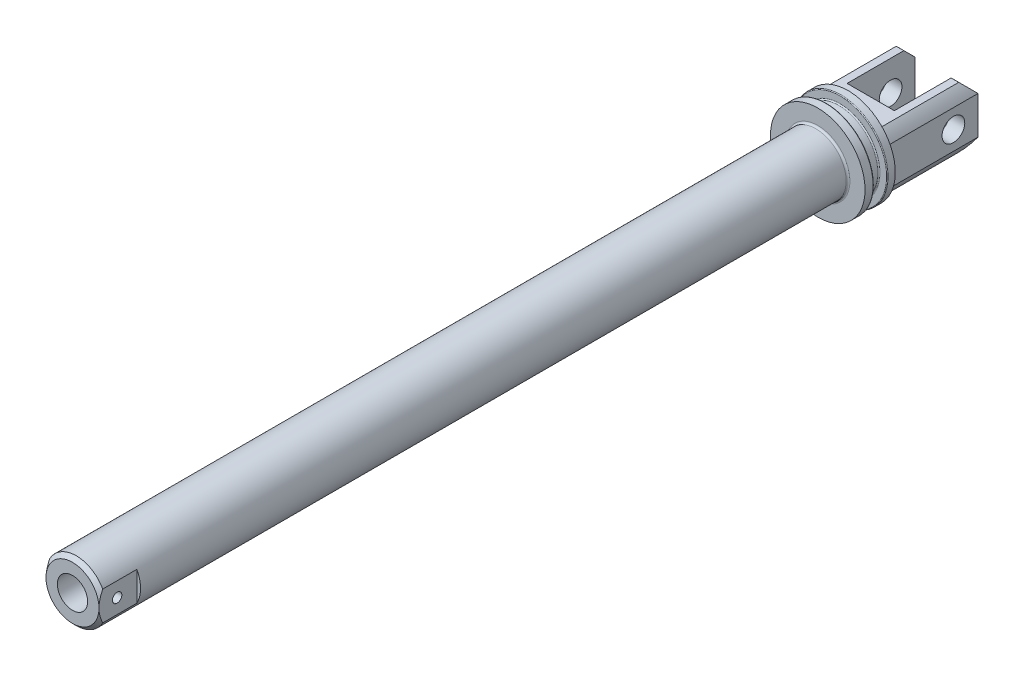
SolidWorks part; units mm, degrees
ref_plane "Front Plane" through (0, 0, 0) normal (0, 0, 1) x (1, 0, 0)
ref_plane "Top Plane" through (0, 0, 0) normal (0, 1, 0) x (1, 0, 0)
ref_plane "Right Plane" through (0, 0, 0) normal (1, 0, 0) x (0, 0, -1)
sketch "Sketch1" plane through (0, 0, 0) normal (0, 0, 1) x (1, 0, 0)
  circle A0 centre (0, 0) radius 8
extrude "Boss-Extrude1" add sketch "Sketch1" along normal blind 197
sketch "Sketch2" plane through (0, 0, 0) normal (0, 0, -1) x (-1, 0, 0)
  circle A0 centre (0, 0) radius 12.5
extrude "Boss-Extrude2" add sketch "Sketch2" along normal blind 8
sketch "Sketch3" plane through (0, 0, 0) normal (0, 1, 0) x (1, 0, 0)
  line L0 (-12.5, 8) -> (-12.5, 0) construction
  line L1 (-12.5, 5.9) -> (-10.25, 5.9)
  line L2 (-12.5, 5.9) -> (-12.5, 2.3)
  line L3 (-12.5, 2.3) -> (-10.25, 2.3)
  line L4 (-10.25, 5.9) -> (-10.25, 2.3)
  line L5 (12.5, 8) -> (-12.5, 8) construction
  line L6 (0, 10.0082) -> (0, -3.7228) construction
  dimension "D1" = 3.6
  dimension "D2" = 2.1
  dimension "D3" = 2.25
revolve "Cut-Revolve1" cut sketch "Sketch3" angle 360 about L6
sketch "Sketch8" plane through (0, 0, -8) normal (0, 0, -1) x (-1, 0, 0)
  circle A0 centre (0, 0) radius 11.5
extrude "Boss-Extrude4" add sketch "Sketch8" along normal blind 24
sketch "Sketch10" plane through (0, 0, 0) normal (0, 1, 0) x (1, 0, 0)
  line L0 (0, 37.7371) -> (0, 5.0633) construction
  line L1 (11.5, 32) -> (-11.5, 32) construction
  line L2 (-6.25, 35.6058) -> (6.25, 35.6058)
  line L3 (-6.25, 35.6058) -> (-6.25, 14)
  line L4 (-6.25, 14) -> (6.25, 14)
  line L5 (6.25, 35.6058) -> (6.25, 14)
  line L6 (-6.25, 35.6058) -> (6.25, 14) construction
  line L7 (-6.25, 14) -> (6.25, 35.6058) construction
  point P3 (0, 24.8029)
  dimension "D1" = 18
  dimension "D2" = 12.5
extrude "Cut-Extrude1" cut sketch "Sketch10" against normal through all both and the other way through all
sketch "Sketch13" plane through (0, 0, -32) normal (0, 0, -1) x (-1, 0, 0)
  line L0 (10.3562, -5) -> (10.3562, 5)
  line L9 (11, 5) -> (10.3562, 4.7073) construction
  line L10 (10.4692, -4.7587) -> (10.3562, -4.7073) construction
  line L11 (-10.3562, -5) -> (-10.3562, 5)
  arc A0 (-10.3562, 5) -> (-10.3562, -5) centre (0, 0) ccw
  arc A1 (10.3562, -5) -> (10.3562, 5) centre (0, 0) ccw
  point P0 (0, 0)
  point P1 (0, 0)
sketch "Sketch11" plane through (0, -11.5, -32) normal (-1, 0, 0) x (0, 0, -1)
  line L1 (-32, -11.5) -> (13.2543, -11.5) construction
  line L7 (1.4984, -3.5) -> (-24, -19.5) construction
  line L8 (1.4984, -19.5) -> (-24, -3.5) construction
  line L9 (0.011, -16.5) -> (-3, -19.5)
  line L11 (-24, -19.5) -> (-24, -26.3966)
  line L12 (-24, -26.3966) -> (1.4984, -26.3966)
  line L13 (1.4984, -19.5) -> (1.4984, -26.3966)
  line L15 (-24, -3.5) -> (-24, 3.3597)
  line L16 (-24, 3.3597) -> (2.7695, 3.3597)
  line L17 (2.7695, -3.5) -> (2.7695, 3.3597)
  line L18 (0, -21.1534) -> (0, -1.8466) construction
  line L19 (1.4984, -19.5) -> (0.011, -19.5)
  line L20 (0.011, -19.5) -> (0.011, -16.5)
  line L21 (-3, -19.5) -> (-24, -19.5)
  line L22 (-3, -3.5) -> (-24, -3.5)
  line L23 (0.011, -6.5) -> (-3, -3.5)
  line L24 (0.011, -3.5) -> (0.011, -6.5)
  line L25 (1.4984, -3.5) -> (0.011, -3.5)
  line L26 (1.4984, -3.5) -> (2.7695, -3.5)
  point P0 (-11.2508, -11.5)
  dimension "D1" = 3
  dimension "D2" = 16
  dimension "D3" = 3
extrude "Cut-Extrude3" cut sketch "Sketch11" against normal through all both and the other way through all
extrude "Cut-Extrude5" cut sketch "Sketch13" against normal blind 24
fillet "Fillet1" radius 0.5 1 edges at (8, 0, 0)
fillet "Fillet2" radius 0.2 2 edges at (-12.5, 0, -5.9) (-12.5, 0, -2.3)
fillet "Fillet3" radius 0.3 2 edges at (-10.25, 0, -2.3) (-10.25, 0, -5.9)
chamfer "Chamfer3" distance 1 angle 45 1 edges at (8, 0, 197)
sketch "Sketch15" plane through (0, 8, 0) normal (0, 1, 0) x (1, 0, 0)
  line L0 (8, -196) -> (8, -0.5) construction
  line L1 (-7, -187) -> (-9.1993, -187)
  line L2 (-7, -187) -> (-7, -197)
  line L3 (-7, -197) -> (-9.1993, -197)
  line L4 (-9.1993, -187) -> (-9.1993, -197)
  line L5 (-8.5, -153.05) -> (-9.4702, -153.05)
  line L6 (-6, -155.55) -> (-6, -175.45)
  line L7 (-8.5, -177.95) -> (-9.4702, -177.95)
  line L8 (-9.4702, -153.05) -> (-9.4702, -177.95)
  line L9 (-8, -197) -> (8, -197) construction
  line L10 (9.8801, -187) -> (7, -187)
  line L11 (9.8801, -187) -> (9.8801, -197)
  line L12 (9.8801, -197) -> (7, -197)
  line L13 (7, -187) -> (7, -197)
  line L14 (-8, -0.5) -> (-8, -196) construction
  arc A0 (-8.5, -177.95) -> (-6, -175.45) centre (-8.5, -175.45) ccw
  arc A1 (-8.5, -153.05) -> (-6, -155.55) centre (-8.5, -155.55) cw
  dimension "D10" = 2.5
  dimension "D1" = 24.9
  dimension "D2" = 10
  dimension "D3" = 14
  dimension "D4" = 10
  dimension "D5" = 10
  dimension "D6" = 0
  dimension "D7" = 14
  dimension "D8" = 1
  dimension "D9" = 19.05
extrude "Cut-Extrude7" cut sketch "Sketch15" against normal through all both and the other way through all
sketch "Sketch14" plane through (10.3562, 0, 0) normal (1, 0, 0) x (0, 0, -1)
  line L0 (32, -5) -> (32, 5) construction
  circle A0 centre (25.5, 0) radius 3
  dimension "D1" = 6.5
extrude "Cut-Extrude6" cut sketch "Sketch14" against normal blind 24
sketch "Sketch16" plane through (7, 0, 0) normal (1, 0, 0) x (0, 0, -1)
  line L0 (-196, -8) -> (-0.5, -8) construction
  line L1 (-197, 7) -> (-197, 0) construction
  circle A0 centre (-192.2, 0) radius 0.6474
  dimension "D1" = 8
  dimension "D2" = 4.8
hole_wizard "Hole2" positions "Sketch18" profile "Sketch19" legacy
sketch "Sketch18" plane through (0, 0, 197) normal (0, 0, 1) x (1, 0, 0)
  point P0 (0, 0)
sketch "Sketch19" plane through (0, 0, 197) normal (1, 0, 0) x (0, -1, 0)
  line L0 (0, 0) -> (0, 7.5)
  line L1 (0, 7.5) -> (4, 7.5)
  line L2 (4, 7.5) -> (4, 0)
  line L3 (4, 0) -> (0, 0)
  line L4 (0, 110) -> (0, -10) construction
  dimension "直径" = 8
  dimension "深度" = 7.5
hole_wizard "M6 Tapped Hole1" positions "Sketch20" profile "Sketch21" tap size "M6" standard "GB"
sketch "Sketch20" plane through (0, 0, 197) normal (0, 0, 1) x (1, 0, 0)
  point P0 (0, 0)
sketch "Sketch21" plane through (0, 0, 197) normal (1, 0, 0) x (0, -1, 0)
  line L0 (0, 0) -> (0, 19.5022)
  line L1 (0, 19.5022) -> (2.5, 18)
  line L2 (2.5, 18) -> (2.5, 0)
  line L5 (2.5, 0) -> (0, 0)
  line L10 (0, 19.5022) -> (-2.5, 18) construction
  line L11 (0, -6.35) -> (0, 107.95) construction
  dimension "螺纹孔钻头直径" = 5
  dimension "螺纹孔钻头深度" = 18
  dimension "导头角度" = 118
cosmetic thread "Cosmetic Thread1" parameters "D1"=12, "D2"=6
hole_wizard "M3 Tapped Hole1" positions "Sketch22" profile "Sketch23" tap size "M3" standard "GB"
sketch "Sketch22" plane through (7, 0, 0) normal (1, 0, 0) x (0, 0, -1)
  point P0 (-192.2, 0)
sketch "Sketch23" plane through (7, 0, 192.2) normal (0, 1, 0) x (0, 0, -1)
  line L0 (0, 0) -> (0, 8.2511)
  line L1 (0, 8.2511) -> (1.25, 7.5)
  line L2 (1.25, 7.5) -> (1.25, 0)
  line L5 (1.25, 0) -> (0, 0)
  line L10 (0, 8.2511) -> (-1.25, 7.5) construction
  line L11 (0, -6.35) -> (0, 107.95) construction
  dimension "螺纹孔钻头直径" = 2.5
  dimension "螺纹孔钻头深度" = 7.5
  dimension "导头角度" = 118
cosmetic thread "Cosmetic Thread2" parameters "D1"=3.2003, "D2"=3
